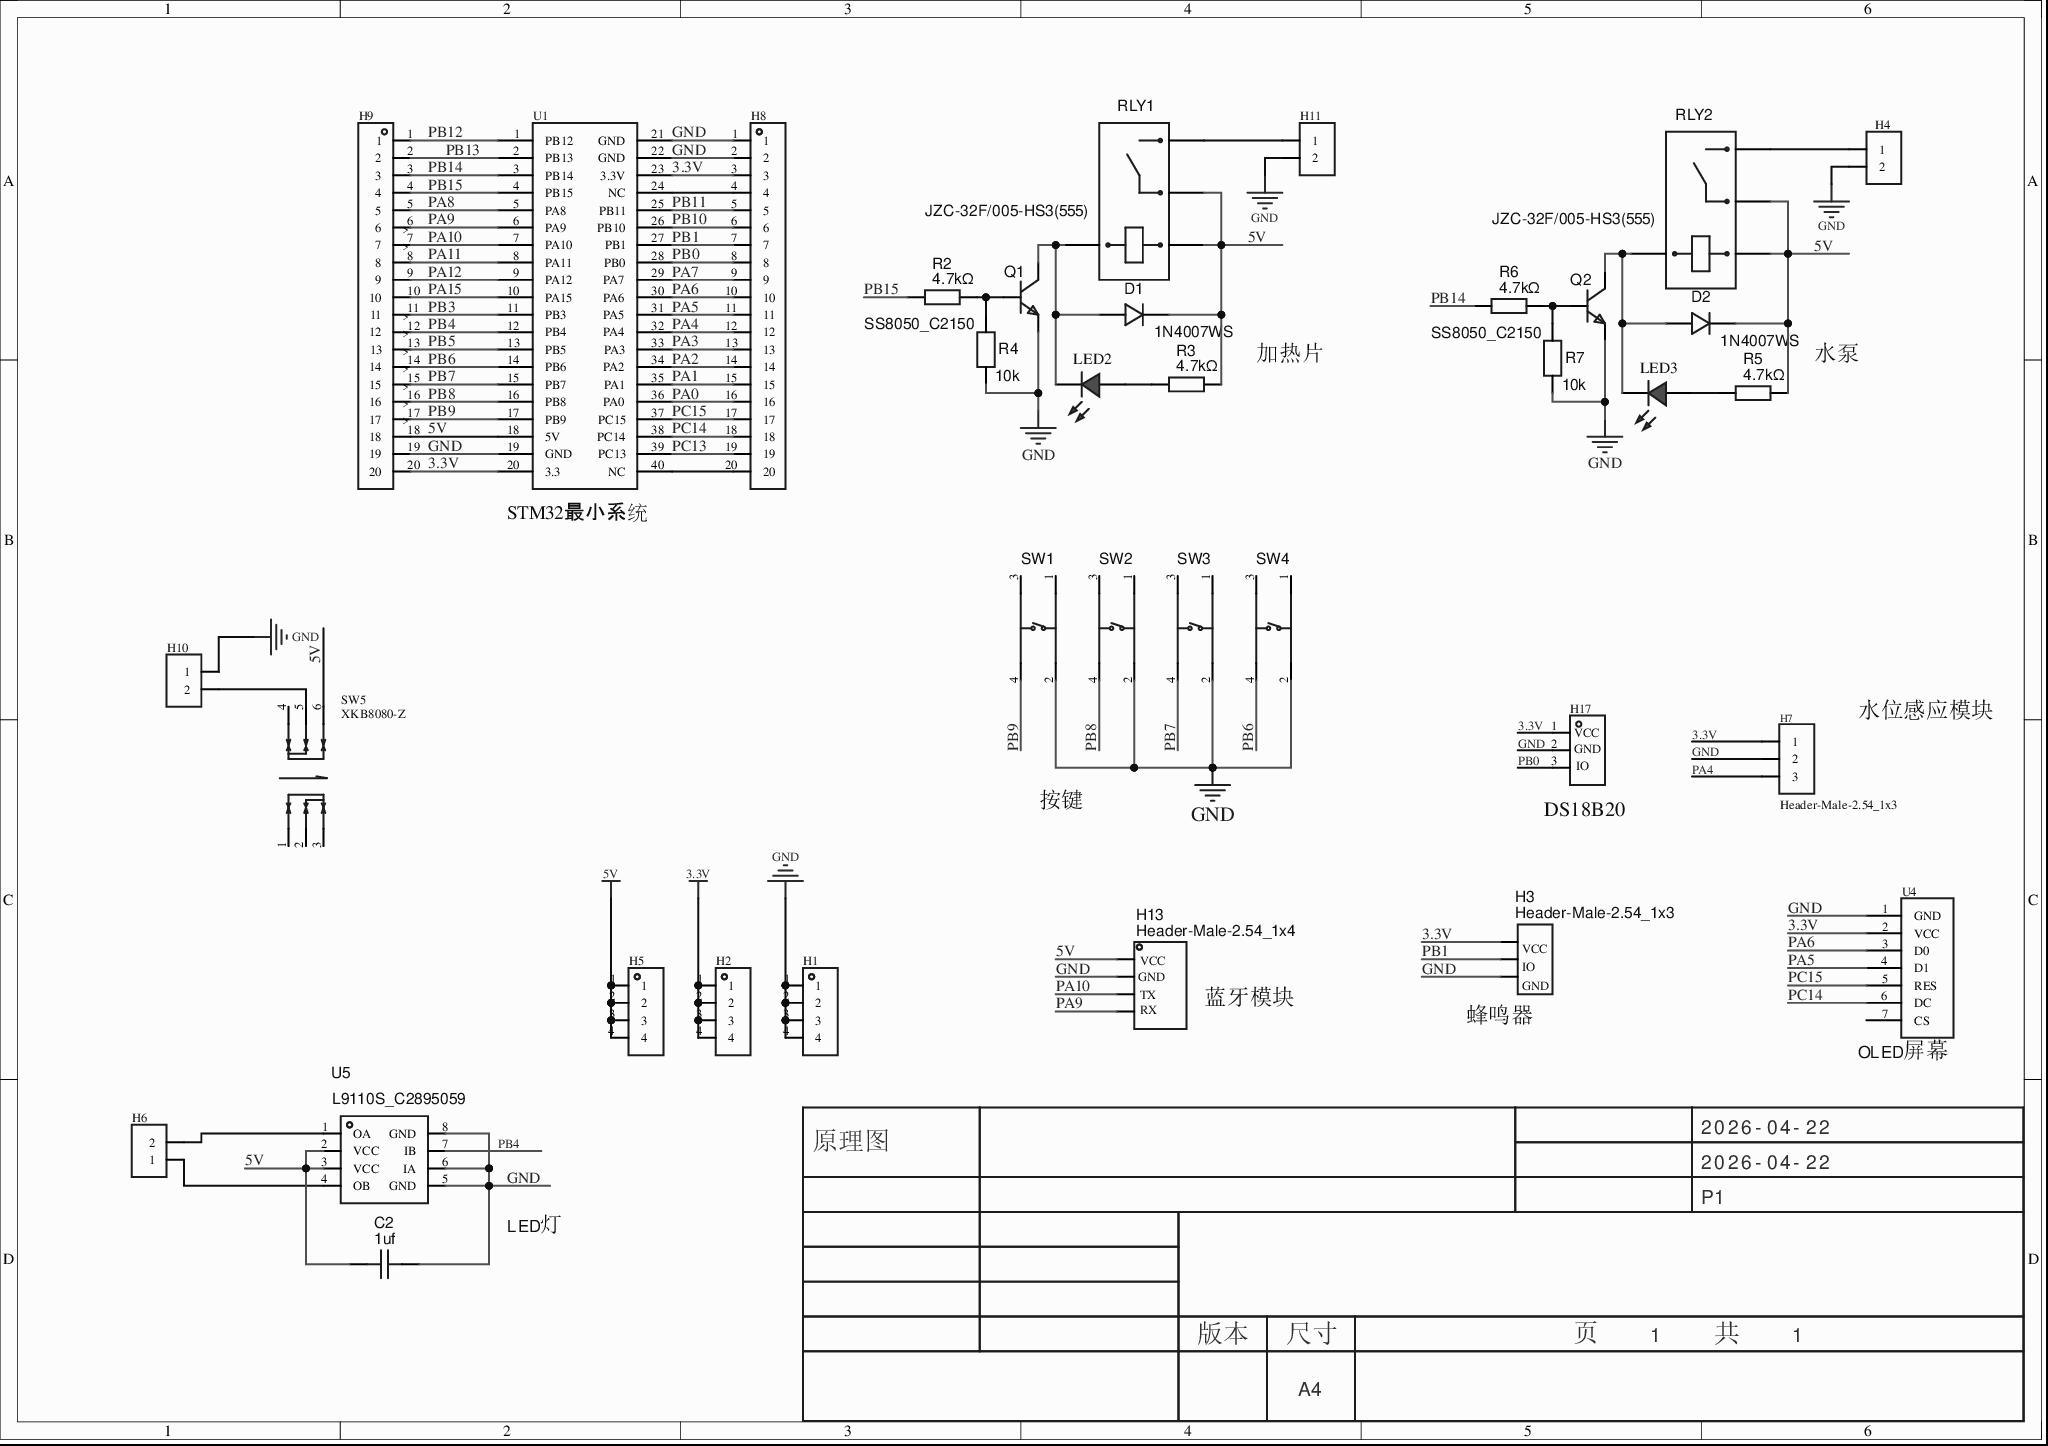
[diagram p0: MISC51992-3.schdoc]
# Altium project MISC51992-2.PrjPcb
1 sheet, 36 parts. Net scope: global (net labels, ports and power ports of the same name join across sheets).
Board file: MISC51992.pcbdoc

## Sheet MISC51992-3.schdoc
size 297 x 209 mm; Version: V1.0; @Project Name: MISC51992; @Page Count: 1; @Update Date: 2026-04-22; @Create Date: 2026-04-22; @Schematic Name: MISC51992; @Page No: 1; @Create Time: 18:45:31; @Update Time: 18:45:31; @Board Name: MISC51992

### Parts
C2  1uf  [C0805]
D1  1N4007WS  [SOD-323_L1.8-W1.3-LS2.5-RD]
D2  1N4007WS  [SOD-323_L1.8-W1.3-LS2.5-RD]
H1  (no value)  [HDR-TH_4P-P2.54-V-F]
H2  (no value)  [HDR-TH_4P-P2.54-V-F]
H3  Header-Male-2.54_1x3  [HDR-TH_3P-P2.54-V-M-1]
H4  (no value)  [HDR-TH_2P-P2.54-V-F]
H5  (no value)  [HDR-TH_4P-P2.54-V-F]
H6  (no value)  [HDR-TH_2P-P2.54-V-F]
H7  Header-Male-2.54_1x3  [HDR-TH_3P-P2.54-V-M-1]
H8  (no value)  [HDR-TH_20P-P2.54-V-M-1]
H9  (no value)  [HDR-TH_20P-P2.54-V-M-1]
H10  (no value)  [HDR-TH_2P-P2.54-V-F]
H11  (no value)  [HDR-TH_2P-P2.54-V-F]
H13  Header-Male-2.54_1x4  [HDR-TH_4P-P2.54-V-M]
H17  (no value)  [HDR-TH_3P-P2.54-V-F]
LED2  (no value)  [LED_0805]
LED3  (no value)  [LED_0805]
Q1  SS8050_C2150  [SOT-23-3_L2.9-W1.3-P1.90-LS2.4-BR]
Q2  SS8050_C2150  [SOT-23-3_L2.9-W1.3-P1.90-LS2.4-BR]
R2  4.7kΩ  [R0805]
R3  4.7kΩ  [R0805]
R4  10k  [R0805]
R5  4.7kΩ  [R0805]
R6  4.7kΩ  [R0805]
R7  10k  [R0805]
RLY1  JZC-32F/005-HS3(555)  [RELAY-TH_JZC-32F-XXXHXX]
RLY2  JZC-32F/005-HS3(555)  [RELAY-TH_JZC-32F-XXXHXX]
SW1  TS665CJ  [SW-TH_4P-L6.0-W6.0-P4.50-LS6.5]  (value not drawn)
SW2  TS665CJ  [SW-TH_4P-L6.0-W6.0-P4.50-LS6.5]  (value not drawn)
SW3  TS665CJ  [SW-TH_4P-L6.0-W6.0-P4.50-LS6.5]  (value not drawn)
SW4  TS665CJ  [SW-TH_4P-L6.0-W6.0-P4.50-LS6.5]  (value not drawn)
SW5  XKB8080-Z  [SW-TH_6P-L8.0-W8.0-P2.50]
U1  (no value)  [STM32最小系统]
U4  (no value)  [OLED12864/7针]
U5  L9110S_C2895059  [SOP-8_L5.0-W4.0-P1.27-LS6.0-BL]

### Nets
3.3V: H2.1 H2.2 H2.3 H2.4 H3.1 H7.1 H8.3 H9.20 H17.1 U1.20(3.3) U1.23(3.3V) U4.2(VCC)
5V: C2.1 D1.1(K) D2.1(K) H5.1 H5.2 H5.3 H5.4 H9.18 H13.1 R3.2 R5.2 RLY1.1 RLY1.4 RLY2.1 RLY2.4 SW5.6 U1.18(5V) U5.2(VCC) U5.3(VCC)
GND: C2.2 H1.1 H1.2 H1.3 H1.4 H3.3 H4.2 H7.2 H8.1 H8.2 H9.19 H10.1 H11.2 H13.2 H17.2 Q1.2(E) Q2.2(E) R4.1 R7.1 SW1.2(B) SW2.2(B) SW3.2(B) SW4.2(B) U1.19(GND) U1.21(GND) U1.22(GND) U4.1(GND) U5.5(GND) U5.6(IA) U5.8(GND)
PA0: H8.16 U1.36(PA0)
PA1: H8.15 U1.35(PA1)
PA2: H8.14 U1.34(PA2)
PA3: H8.13 U1.33(PA3)
PA4: H7.3 H8.12 U1.32(PA4)
PA5: H8.11 U1.31(PA5) U4.4(D1)
PA6: H8.10 U1.30(PA6) U4.3(D0)
PA7: H8.9 U1.29(PA7)
PA8: H9.5 U1.5(PA8)
PA9: H9.6 H13.4 U1.6(PA9)
PA10: H9.7 H13.3 U1.7(PA10)
PA11: H9.8 U1.8(PA11)
PA12: H9.9 U1.9(PA12)
PA15: H9.10 U1.10(PA15)
PB0: H8.8 H17.3 U1.28(PB0)
PB1: H3.2 H8.7 U1.27(PB1)
PB3: H9.11 U1.11(PB3)
PB4: H9.12 U1.12(PB4) U5.7(IB)
PB5: H9.13 U1.13(PB5)
PB6: H9.14 SW4.4(D) U1.14(PB6)
PB7: H9.15 SW3.4(D) U1.15(PB7)
PB8: H9.16 SW2.4(D) U1.16(PB8)
PB9: H9.17 SW1.4(D) U1.17(PB9)
PB10: H8.6 U1.26(PB10)
PB11: H8.5 U1.25(PB11)
PB12: H9.1 U1.1(PB12)
PB13: H9.2 U1.2(PB13)
PB14: H9.3 R6.1 U1.3(PB14)
PB15: H9.4 R2.1 U1.4(PB15)
PC13: H8.19 U1.39(PC13)
PC14: H8.18 U1.38(PC14) U4.6(DC)
PC15: H8.17 U1.37(PC15) U4.5(RES)
NetD1_2: D1.2(A) LED2.1(C) Q1.3(C) RLY1.2
NetD2_2: D2.2(A) LED3.1(C) Q2.3(C) RLY2.2
NetH4_1: H4.1 RLY2.3
NetH6_1: H6.1 U5.4(OB)
NetH6_2: H6.2 U5.1(OA)
NetH8_4: H8.4 U1.24(NC)
NetH8_20: H8.20 U1.40(NC)
NetH10_2: H10.2 SW5.5
NetH11_1: H11.1 RLY1.3
NetLED2_2: LED2.2(A) R3.1
NetLED3_2: LED3.2(A) R5.1
NetQ1_1: Q1.1(B) R2.2 R4.2
NetQ2_1: Q2.1(B) R6.2 R7.2

Not connected (* = marked no-connect by the designer): SW1 1(A)* 3(C)*; SW2 1(A)* 3(C)*; SW3 1(A)* 3(C)*; SW4 1(A)* 3(C)*; SW5 1 2 3 4; U4 7(CS)*

### Notes on the sheet
- (near H9) >
- (near R3) 加热片
- (near R5) 水泵
- (near U1) STM32最小系统
- (near H17) GND
- (near H17) VCC
- (near H17) IO
- 水位感应模块
- 按键
- (near H17) DS18B20
- (near H3) VCC
- (near H13) GND
- (near H13) RX
- (near H13) TX
- (near H13) VCC
- 蓝牙模块
- (near H3) 蜂鸣器
- (near H3) GND
- (near H3) IO
- (near U4) OLED屏幕
- LED灯
- 2026-04-22
- 原理图
- P1
- 版本
- 尺寸
- A4
- 页    1    共    1

### Library data of the parts
C2 = 1uf: Add into BOM: yes; Symbol: 1uf; Device: 1uf; Convert to PCB: yes; Origin Footprint: C0805; FootprintName: C0805
D1 D2 = 1N4007WS: Manufacturer: MDD; Add into BOM: yes; ModelId: db63db13d9e342eb939127d413d6200b; Symbol: 1N4007WS; Device: 1N4007WS; Convert to PCB: yes; Origin Footprint: SOD-323_L1.8-W1.3-LS2.5-RD; Supplier: LCSC; Supplier Part: C193404; Manufacturer Part: 1N4007WS; JLCPCB Part Class: Extended Part; FootprintName: SOD-323_L1.8-W1.3-LS2.5-RD; ModelName: SOD-323_L1.8-W1.3-LS2.5-RD
H1 H2 H5 = HDR-F_2.54_1x4P: Symbol: 2.54-1*4P母; 3D Model: d187812051054f85879fcaa51a310d8e0819f05c4eef4c71ace90d822a990e87; 3D Model Transform: 419.6842,98.464,0,0,0,0,0,0,-118.11; ConvertToPcb: yes; Device: HDR-F_2.54_1x4P; Supplier Part: C2718488; Supplier Footprint: 插件; AddInBom: yes; FootprintName: HDR-TH_4P-P2.54-V-F; ModelName: HDR-TH_4P-P2.54-V-F
H3 = Header-Male-2.54_1x3: Manufacturer: BOOMELE; Manufacturer Part: Header2.54mm 1*3P; Add into BOM: yes; Symbol: Header-Male-2.54_1x3; Device: Header-Male-2.54_1x3; Convert to PCB: yes; Origin Footprint: HDR-TH_3P-P2.54-V-M-1; Supplier: LCSC; Supplier Part: C49257; JLCPCB Part Class: Extended Part; FootprintName: HDR-TH_3P-P2.54-V-M-1
H4 H6 H10 H11 = HDR-F_2.54_1x2P: Symbol: Header-Female-2.54_1x2; 3D Model: a9450ef445564560a104363b9aacde4e; 3D Model Transform: 215.7476,98.425,0,0,0,0,0,0,-129.921; ConvertToPcb: yes; ModelName: HDR-TH_2P-P2.54-F-LI-1X2P; Device: HDR-F_2.54_1x2P; Supplier Part: C49661; Supplier Footprint: 插件; AddInBom: yes; FootprintName: HDR-TH_2P-P2.54-V-F
H7 = Header-Male-2.54_1x3: Manufacturer: BOOMELE; Manufacturer Part: Header2.54mm 1*3P; ConvertToPcb: yes; Symbol: Header-Male-2.54_1x3; Device: Header-Male-2.54_1x3; Supplier: LCSC; Supplier Part: C49257; JLCPCB Part Class: Extended Part; AddInBom: yes; FootprintName: HDR-TH_3P-P2.54-V-M-1
H8 H9 = HDR-M_2.54_1x20P: 间距:2.54mm;总PIN位数:20;排数:1;插针结构:-;行距:-;安装类型:直插;圆针/方针:-;额定电流:-;额定电压:-;配合针长度:-;塑高:-;触头材质:黄铜;触头镀层:-;颜色:黑色;; Symbol: HDR_2.54-1x20P; ConvertToPcb: yes; ModelId: f68709be121d406db68b06f32a5953890819f05c4eef4c71ace90d822a990e87; ModelName: HDR-M-2.54_1x20; ModelTransform: 1999.996,100,0,0,0,0,0,2.48,-118.11; Device: HDR-M_2.54_1x20P; AddInBom: yes; SupplierPart: C50981; Supplier Footprint: 插件; FootprintName: HDR-TH_20P-P2.54-V-M-1
H13 = Header-Male-2.54_1x4: Manufacturer: Ckmtw; Manufacturer Part: 210S-1*4P L=11.6MMGold-plated black; Add into BOM: yes; ModelId: 1d5b704bd9074887b1bc895e6ed65ccf; Symbol: Header-Male-2.54_1x4; Device: Header-Male-2.54_1x4; Convert to PCB: yes; Origin Footprint: HDR-TH_4P-P2.54-V-M; Supplier: LCSC; Supplier Part: C124378; JLCPCB Part Class: Extended Part; FootprintName: HDR-TH_4P-P2.54-V-M; ModelName: HDR-TH_4P-P2.54-V-M
H17 = HDR-F_2.54_1x3P: Symbol: PM254V-11-03-H85; 3D Model: f3b3cc5aae9641bf9e56fc160cef875b0819f05c4eef4c71ace90d822a990e87; 3D Model Transform: 299.9994,100,0,0,0,0,0,0,-118.11; ConvertToPcb: yes; ModelName: HDR2.54-F-LI-1X3P; Device: HDR-F_2.54_1x3P; Supplier Part: C541850; Supplier Footprint: 插件; AddInBom: yes; FootprintName: HDR-TH_3P-P2.54-V-F
LED2 LED3 = LED_0805-R: Symbol: LED_R; Convert to PCB: yes; 3D Model: 33fb9fca58e84f37a403ebeef4c28b77; 3D Model Transform: 78.7,49.1,39.3,0,0,0,0,0,0; ModelName: LED-0805_R; Device: LED_0805-R; Add into BOM: yes; Supplier Footprint: 0805; FootprintName: LED_0805
Q1 Q2 = SS8050_C2150: Manufacturer: CJ(江苏长电/长晶); Manufacturer Part: SS8050; Add into BOM: yes; Symbol: SS8050_C2150; Device: SS8050_C2150; Convert to PCB: yes; Origin Footprint: SOT-23-3_L2.9-W1.3-P1.90-LS2.4-BR; Supplier: LCSC; Supplier Part: C2150; JLCPCB Part Class: Basic Part; FootprintName: SOT-23-3_L2.9-W1.3-P1.90-LS2.4-BR
R2 R3 R5 R6 = 4.7kΩ: Manufacturer: UNI-ROYAL(厚声); Manufacturer Part: 0805W8F4701T5E; Add into BOM: yes; Resistance: 4.7K; ModelId: 1f8f9bfd8e2b427398b06535d781678a; Symbol: 4.7kΩ; Device: 4.7kΩ; Convert to PCB: yes; Origin Footprint: R0805; Supplier: LCSC; Supplier Part: C17673; JLCPCB Part Class: Basic Part; FootprintName: R0805; ModelName: R0805
R4 R7 = 51k: Add into BOM: yes; ModelId: 1f8f9bfd8e2b427398b06535d781678a; Symbol: 51k; Device: 51k; Convert to PCB: yes; Origin Footprint: R0805; FootprintName: R0805; ModelName: R0805
RLY1 RLY2 = JZC-32F/005-HS3(555): Manufacturer: HF(宏发); Add into BOM: yes; Symbol: JZC-32F/005-HS3(555); Device: JZC-32F/005-HS3(555); Convert to PCB: yes; Origin Footprint: RELAY-TH_JZC-32F-XXXHXX; Supplier: LCSC; Manufacturer Part: JZC-32F/005-HS3(555); Supplier Part: C9222; JLCPCB Part Class: Extended Part; FootprintName: RELAY-TH_JZC-32F-XXXHXX
SW1-SW4 = TS665CJ: Manufacturer: SHOU HAN; Add into BOM: yes; Symbol: TS665CJ; Device: TS665CJ; Convert to PCB: yes; Origin Footprint: SW-TH_4P-L6.0-W6.0-P4.50-LS6.5; Supplier: LCSC; Supplier Part: C393938; Manufacturer Part: TS665CJ; JLCPCB Part Class: Extended Part; FootprintName: SW-TH_4P-L6.0-W6.0-P4.50-LS6.5
SW5 = XKB8080-Z: 自锁/无锁:自锁;安装方式:直插;触点电流:100mA;额定电压:30V;带灯:不带;作用力:1.6N;工作寿命:10万次;; Manufacturer: XKB Connection(中国星坤); 3D Model: 2ca63b555ed647238a13c4f5c29203120819f05c4eef4c71ace90d822a990e87; 3D Model Transform: 314.96,314.96,0,90,0,0,0,0,-125.984; Self Lock / No Lock: 自锁; Actuator Style: 矩形按钮; Contact Current: 100mA; Voltage Rating: 30V; Actuator/Cap Color: 蓝色; With Lamp: 不带; Operating Force: 1.6N; Life: 10万次; AddInBom: yes; ModelName: SW-TH_L8.0-W8.0-H13.7-P2.5; Symbol: XKB8080-Z; Device: XKB8080-Z; LCSC Part Name: 8*8 蓝白黑 自锁开关; Supplier Part: C318860; Manufacturer Part: XKB8080-Z; Supplier Footprint: 插件; JLCPCB Part Class: Extended Part; Datasheet: https://item.szlcsc.com/datasheet/XKB8080-Z/299952.html; Supplier: LCSC; IP Rating: -; Mounting Type: 直插; Termination Style: PC引脚; Operating Temperature: -15℃~+55℃; ConvertToPcb: yes; FootprintName: SW-TH_6P-L8.0-W8.0-P2.50
U1 = STM32最小系统: AddInBom: yes; Symbol: STM32最小系统; Device: STM32最小系统; FootprintName: STM32最小系统; ConvertToPcb: yes; Description: STM32最小系统
U4 = OLED12864/7针: AddInBom: yes; Symbol: OLED12864/7针; Device: OLED12864/7针; FootprintName: OLED12864/7针; ConvertToPcb: yes; Description: OLED12864/7针
U5 = L9110S_C2895059: Manufacturer: HTCSEMI(海天芯); Manufacturer Part: L9110S; Add into BOM: yes; Symbol: L9110S_C2895059; Device: L9110S_C2895059; Convert to PCB: yes; Origin Footprint: SOP-8_L5.0-W4.0-P1.27-LS6.0-BL; Supplier: LCSC; Supplier Part: C2895059; JLCPCB Part Class: Extended Part; FootprintName: SOP-8_L5.0-W4.0-P1.27-LS6.0-BL